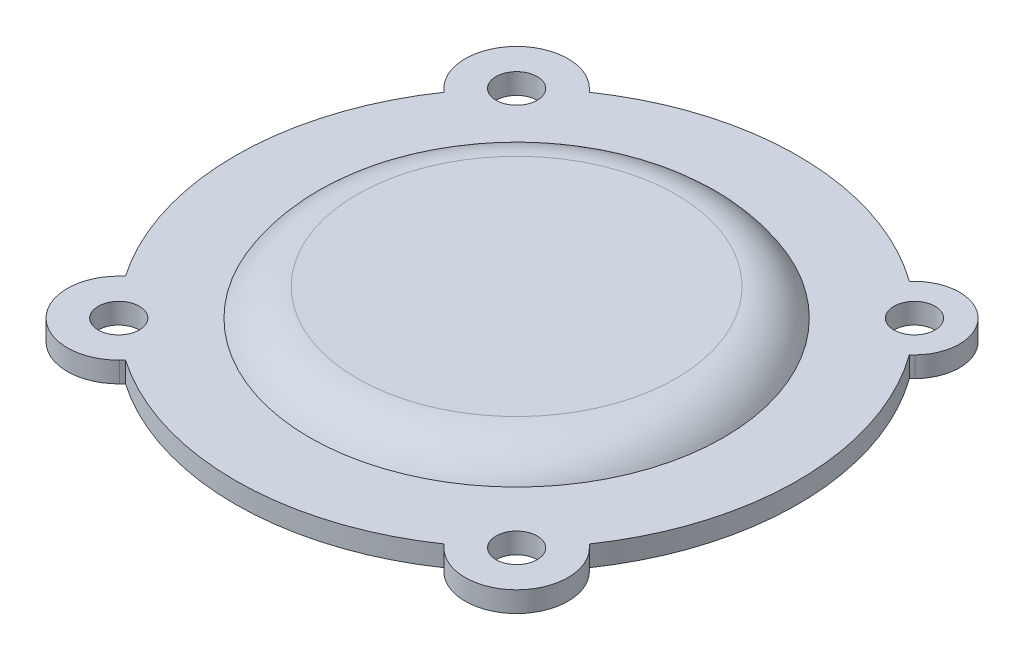
SolidWorks part; units mm, degrees
ref_plane "前视基准面" through (0, 0, 0) normal (0, 0, 1) x (1, 0, 0)
ref_plane "上视基准面" through (0, 0, 0) normal (0, 1, 0) x (1, 0, 0)
ref_plane "右视基准面" through (0, 0, 0) normal (1, 0, 0) x (0, 0, -1)
sketch "草图1" plane through (0, 0, 0) normal (1, 0, 0) x (0, 0, -1)
  line L0 (0, 53.9409) -> (0, -47.9982) construction
  line L2 (0, 12) -> (23.233, 12)
  line L3 (28, 0) -> (31, 0)
  line L4 (31, 0) -> (31, 5)
  line L5 (31, 5) -> (41, 5)
  line L6 (41, 5) -> (41, 8)
  line L7 (41, 8) -> (30.1612, 8)
  line L8 (28, 0) -> (27.1722, 4.6946)
  line L9 (21.201, 8) -> (0, 8)
  line L10 (23.233, 8) -> (21.201, 8)
  line L11 (0, 8) -> (0, 12)
  arc A0 (27.1722, 4.6946) -> (23.233, 8) centre (23.233, 4) ccw
  arc A1 (30.1612, 8) -> (23.233, 12) centre (23.233, 4) ccw
  dimension "D2" = 4
  dimension "D3" = 31
  dimension "D1" = 41
revolve "旋转1" add sketch "草图1" angle 360 about L0
sketch "草图2" plane through (0, 8, 0) normal (0, 1, 0) x (1, 0, 0)
  line L0 (0, 0) -> (50000, 0) construction
  line L1 (0, 0) -> (35355.3391, 35355.3391) construction
  line L2 (0, 0) -> (35355.3391, -35355.3391) construction
  line L3 (-34.2947, 23.6881) -> (-33.8055, 23.1989)
  line L4 (23.9739, 33.2604) -> (24.4062, 33.6829)
  line L5 (34.2943, -23.6877) -> (33.8055, -23.1989)
  line L6 (33.6829, 24.4062) -> (33.2604, 23.9739)
  line L7 (-34.2335, -23.6276) -> (-33.8012, -23.2051)
  line L8 (23.1989, -33.8055) -> (23.6807, -34.2873)
  line L9 (-23.2051, -33.8012) -> (-23.6276, -34.2335)
  line L10 (-23.2036, 33.8022) -> (-23.6429, 34.2491)
  circle A1 centre (0, 0) radius 41 construction
  circle A2 centre (0, 0) radius 35.4595
  arc A5 (-23.6429, 34.2491) -> (-34.2947, 23.6881) centre (-28.9914, 28.9914) ccw
  arc A6 (33.6829, 24.4062) -> (24.4062, 33.6829) centre (28.9914, 28.9914) ccw
  arc A7 (23.6807, -34.2873) -> (34.2943, -23.6877) centre (28.9914, -28.9914) ccw
  arc A8 (-34.2335, -23.6276) -> (-23.6276, -34.2335) centre (-28.9914, -28.9914) ccw
  arc A9 (-33.8055, 23.1989) -> (-33.8012, -23.2051) centre (0, 0) ccw
  arc A10 (23.9739, 33.2604) -> (-23.2036, 33.8022) centre (0, 0) ccw
  arc A11 (33.8055, -23.1989) -> (33.2604, 23.9739) centre (0, 0) ccw
  arc A12 (-23.2051, -33.8012) -> (23.1989, -33.8055) centre (0, 0) ccw
  dimension "D1" = 45
  dimension "D2" = 45
extrude "凸台-拉伸1" add sketch "草图2" against normal blind 3
sketch "草图4" plane through (0, 8, 0) normal (0, 1, 0) x (1, 0, 0)
  circle A0 centre (-28.9914, 28.9914) radius 3
  circle A1 centre (28.9914, 28.9914) radius 3
  circle A2 centre (28.9914, -28.9914) radius 3
  circle A3 centre (-28.9914, -28.9914) radius 3
extrude "切除-拉伸1" cut sketch "草图4" against normal through all
